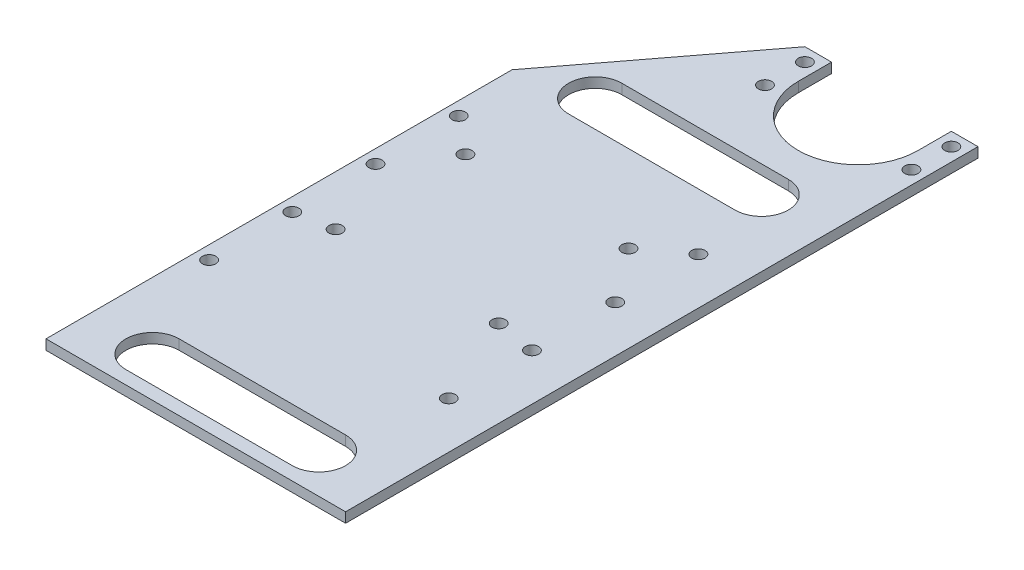
from build123d import *

# Parameters (mm, degrees)
BOSS_EXTRUDE1_DEPTH = 3
SKETCH2_R           = 2
CUT_EXTRUDE1_DEPTH  = 3


with BuildPart() as part:
    # Sketch1 → Boss-Extrude1 (new body)
    with BuildSketch(Plane(origin=(0, 0, 0), x_dir=(1, 0, 0), z_dir=(0, 1, 0))):
        Polygon((-12, -7.26193593), (40, -7.26193593), (40, -197.26193593), (-50, -197.26193593), (-50, -57.26193593), align=None)
    extrude(amount=BOSS_EXTRUDE1_DEPTH)

    # Sketch2 → Cut-Extrude1 (cut)
    with BuildSketch(Plane(origin=(0, 3, 0), x_dir=(1, 0, 0), z_dir=(0, 1, 0))):
        with BuildLine():
            Line((-30, -193.26193593), (20, -193.26193593))
            ThreePointArc((20, -193.26193593), (28, -185.26193593), (20, -177.26193593))
            Line((20, -177.26193593), (-30, -177.26193593))
            ThreePointArc((-30, -177.26193593), (-38, -185.26193593), (-30, -193.26193593))
        make_face()
        with BuildLine():
            Line((-30, -60.26193593), (20, -60.26193593))
            ThreePointArc((20, -60.26193593), (28, -52.26193593), (20, -44.26193593))
            Line((20, -44.26193593), (-30, -44.26193593))
            ThreePointArc((-30, -44.26193593), (-38, -52.26193593), (-30, -60.26193593))
        make_face()
        with BuildLine():
            ThreePointArc((-4, -17.26193593), (14, -35.26193593), (32, -17.26193593))
            Line((32, -17.26193593), (32, -7.26193593))
            Line((32, -7.26193593), (-4, -7.26193593))
            Line((-4, -7.26193593), (-4, -17.26193593))
        make_face()
        with Locations(Location((-46, -152.26193593, 0), (0, 0, 270))):
            Circle(SKETCH2_R)
        with Locations(Location((-46, -77.26193593, 0), (0, 0, 270))):
            Circle(SKETCH2_R)
        with Locations(Location((-46, -127.26193593, 0), (0, 0, 270))):
            Circle(SKETCH2_R)
        with Locations(Location((-46, -102.26193593, 0), (0, 0, 270))):
            Circle(SKETCH2_R)
        with Locations(Location((-8, -11.26193593, 0), (0, 0, 270))):
            Circle(SKETCH2_R)
        with Locations(Location((-8, -23.26193593, 0), (0, 0, 270))):
            Circle(SKETCH2_R)
        with Locations(Location((26, -152.26193593, 0), (0, 0, 270))):
            Circle(SKETCH2_R)
        with Locations(Location((26, -102.26193593, 0), (0, 0, 270))):
            Circle(SKETCH2_R)
        with Locations(Location((26, -127.26193593, 0), (0, 0, 270))):
            Circle(SKETCH2_R)
        with Locations(Location((26, -77.26193593, 0), (0, 0, 270))):
            Circle(SKETCH2_R)
        with Locations(Location((36, -23.26193593, 0), (0, 0, 270))):
            Circle(SKETCH2_R)
        with Locations(Location((36, -11.26193593, 0), (0, 0, 270))):
            Circle(SKETCH2_R)
        with Locations(Location((-35, -86.26193593, 0), (0, 0, 270))):
            Circle(SKETCH2_R)
        with Locations(Location((-35, -125.26193593, 0), (0, 0, 270))):
            Circle(SKETCH2_R)
        with Locations(Location((14, -86.26193593, 0), (0, 0, 270))):
            Circle(SKETCH2_R)
        with Locations(Location((14, -125.26193593, 0), (0, 0, 270))):
            Circle(SKETCH2_R)
    extrude(amount=-CUT_EXTRUDE1_DEPTH, mode=Mode.SUBTRACT)


solid = part.part
